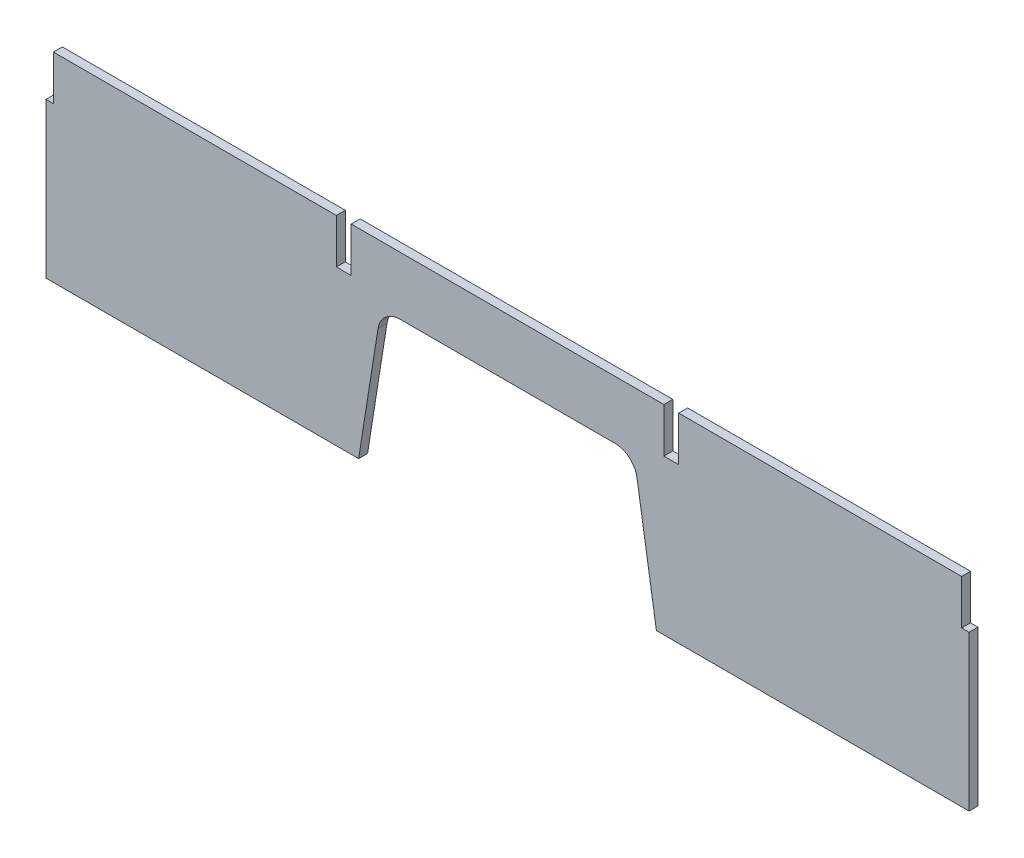
SolidWorks part; units mm, degrees
ref_plane "Front Plane" through (0, 0, 0) normal (0, 0, 1) x (1, 0, 0)
ref_plane "Top Plane" through (0, 0, 0) normal (0, 1, 0) x (1, 0, 0)
ref_plane "Right Plane" through (0, 0, 0) normal (1, 0, 0) x (0, 0, -1)
sketch "Sketch1" plane through (0, 0, 0) normal (0, 0, 1) x (1, 0, 0)
  line L0 (420, 346.7368) -> (420, -168.6127) construction
  line L1 (0, 0) -> (420, 0)
  line L2 (0, 0) -> (0, 208)
  line L3 (10, 268) -> (390, 268)
  line L4 (1240, 0) -> (1240, 208)
  line L5 (820, 462.5943) -> (820, -260.3438) construction
  line L6 (420, 0) -> (446.0848, 164.693)
  line L7 (820, 0) -> (793.9152, 164.693)
  line L8 (475.7155, 190) -> (764.2845, 190)
  line L9 (820, 0) -> (1240, 0)
  line L10 (0, 208) -> (10, 208)
  line L11 (10, 268) -> (10, 208)
  line L12 (390, 268) -> (390, 208)
  line L13 (410, 268) -> (410, 208)
  line L14 (1230, 208) -> (1240, 208)
  line L15 (850, 268) -> (1230, 268)
  line L16 (830, 268) -> (830, 208)
  line L17 (850, 268) -> (850, 208)
  line L18 (1230, 268) -> (1230, 208)
  line L19 (830, 208) -> (850, 208)
  line L20 (410, 268) -> (830, 268)
  line L21 (390, 208) -> (410, 208)
  arc A0 (793.9152, 164.693) -> (764.2845, 190) centre (764.2845, 160) ccw
  arc A1 (446.0848, 164.693) -> (475.7155, 190) centre (475.7155, 160) cw
  dimension "D8" = 30
  dimension "D2" = 1240
  dimension "D3" = 420
  dimension "D4" = 420
  dimension "D5" = 81
  dimension "D6" = 81
  dimension "D7" = 78
  dimension "D9" = 60
  dimension "D10" = 10
  dimension "D11" = 380
  dimension "D12" = 20
  dimension "D13" = 10
  dimension "D14" = 380
  dimension "D15" = 20
  dimension "D16" = 268
extrude "Boss-Extrude1" add sketch "Sketch1" along normal blind 12
